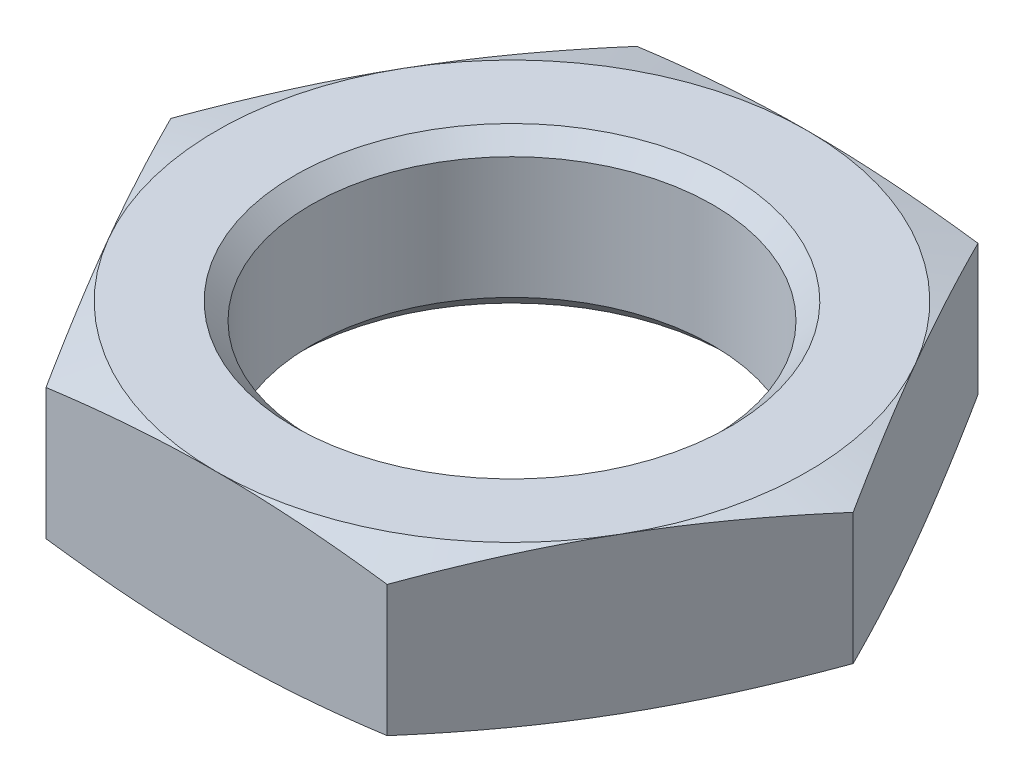
from build123d import *

# Parameters (mm, degrees)
CUT_EXTRUDE1_DEPTH      = 2.5
CUT_EXTRUDE1_DEPTH_BACK = 2.5
SKETCH2_R               = 20


with BuildPart() as part:
    # Sketch1 → Revolve1 (revolve)
    with BuildSketch(Plane.XY, mode=Mode.PRIVATE) as revolve1_sk:
        Polygon((6.4585, -1.9585), (7, -2.5), (9.5, -2.5), (15, -1.026279442), (15, 1.026279442), (9.5, 2.5), (7, 2.5), (6.4585, 1.9585), align=None)
    revolve(revolve1_sk.sketch.rotate(Axis((0, -2.5, 0), (0, 1, 0)), 270), axis=Axis((0, -2.5, 0), (0, 1, 0)))

    # Sketch2 → Cut-Extrude1 (cut, two sides: drawn at the far end of the back side and taken through both)
    with BuildSketch(Plane(origin=(0, 0, 0), x_dir=(1, 0, 0), z_dir=(0, 1, 0)).offset(-CUT_EXTRUDE1_DEPTH_BACK)):
        Circle(SKETCH2_R)
        Polygon((-10.969655115, 0), (-5.484827557, -9.5), (5.484827557, -9.5), (10.969655115, 0), (5.484827557, 9.5), (-5.484827557, 9.5), align=None, mode=Mode.SUBTRACT)
    extrude(amount=CUT_EXTRUDE1_DEPTH + CUT_EXTRUDE1_DEPTH_BACK, mode=Mode.SUBTRACT)


solid = part.part
